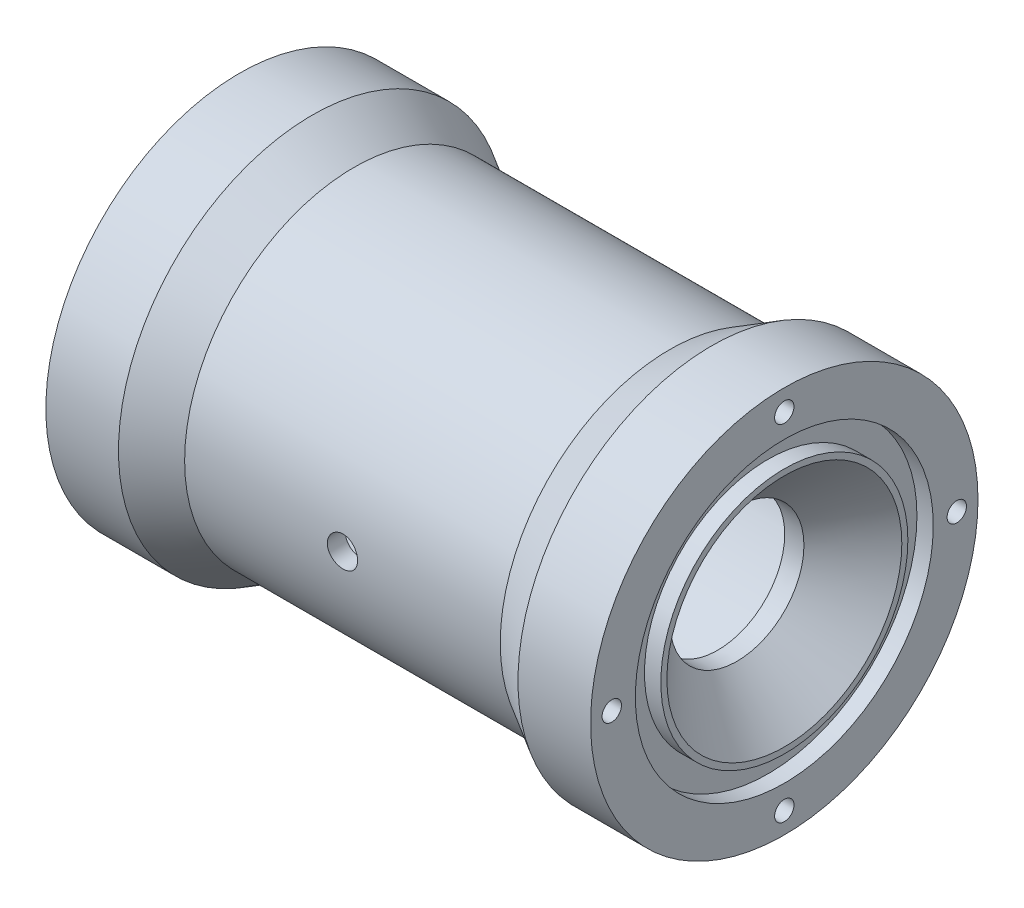
SolidWorks part; units mm, degrees
ref_plane "前视基准面" through (0, 0, 0) normal (0, 0, 1) x (1, 0, 0)
ref_plane "上视基准面" through (0, 0, 0) normal (0, 1, 0) x (1, 0, 0)
ref_plane "右视基准面" through (0, 0, 0) normal (1, 0, 0) x (0, 0, -1)
sketch "草图1" plane through (0, 0, 0) normal (0, 0, 1) x (1, 0, 0)
  line L0 (16.5, 16) -> (13.0359, 14)
  line L1 (22.4976, 16) -> (16.5, 16)
  line L2 (13.0359, 14) -> (-13.0359, 14)
  line L3 (-13.0359, 14) -> (-16.5, 16)
  line L4 (-16.5, 16) -> (-22.5, 16)
  line L5 (22.4976, 16) -> (22.4976, 12.3038)
  line L6 (22.4976, 12.3038) -> (21.1514, 12.3038)
  line L7 (21.1514, 12.3038) -> (21.1514, 10.2038)
  line L8 (21.1514, 10.2038) -> (22.5016, 10.2038)
  line L9 (22.5016, 10.2038) -> (22.5019, 9.7038)
  line L10 (22.5019, 9.7038) -> (18.5923, 5.5284)
  line L11 (18.5923, 5.5284) -> (17.0048, 5.5273)
  line L12 (17.0048, 5.5273) -> (17, 12.5)
  line L13 (17, 12.5) -> (-22.5, 12.5)
  line L14 (-22.5, 12.5) -> (-22.5, 16)
  line L15 (22.5, 0) -> (-22.5, 0) construction
revolve "旋转1" add sketch "草图1" angle 360 about L15
hole_wizard "M2 螺纹孔1" positions "草图2" profile "草图3" tap size "M2" standard "GB"
sketch "草图2" plane through (22.4976, 0, 0) normal (1, 0, 0) x (0, 0, -1)
  point P0 (0, 14.25)
  point P8 (14.25, 0)
  point P9 (0, -14.25)
  point P10 (-14.25, 0)
  point P11 (0, 0)
  dimension "D1" = 14.25
  dimension "D2" = 4
sketch "草图3" plane through (22.4976, 14.25, 0) normal (0, 1, 0) x (0, 0, -1)
  line L0 (0, 0) -> (0, 5.4807)
  line L1 (0, 5.4807) -> (0.8, 5)
  line L2 (0.8, 5) -> (0.8, 0)
  line L5 (0.8, 0) -> (0, 0)
  line L10 (0, 5.4807) -> (-0.8, 5) construction
  line L11 (0, -6.35) -> (0, 107.95) construction
  dimension "螺纹孔钻头直径" = 1.6
  dimension "螺纹孔钻头深度" = 5
  dimension "导头角度" = 118
cosmetic thread "孔螺蚊线1" parameters "D1"=4, "D2"=2
cosmetic thread "孔螺蚊线2" parameters "D1"=4, "D2"=2
cosmetic thread "孔螺蚊线3" parameters "D1"=4, "D2"=2
cosmetic thread "孔螺蚊线4" parameters "D1"=4, "D2"=2
hole_wizard "M2 螺纹孔2" positions "草图4" profile "草图5" tap size "M2" standard "GB"
sketch "草图4" plane through (-22.5, 0, 0) normal (-1, 0, 0) x (0, 0, 1)
  point P0 (0, 14.25)
  point P7 (14.25, 0)
  point P8 (0, -14.25)
  point P9 (-14.25, 0)
  point P10 (0, 0)
  dimension "D1" = 4
sketch "草图5" plane through (-22.5, 14.25, 0) normal (0, 1, 0) x (0, 0, 1)
  line L0 (0, 0) -> (0, 5.6807)
  line L1 (0, 5.6807) -> (0.8, 5.2)
  line L2 (0.8, 5.2) -> (0.8, 0)
  line L5 (0.8, 0) -> (0, 0)
  line L10 (0, 5.6807) -> (-0.8, 5.2) construction
  line L11 (0, -6.35) -> (0, 107.95) construction
  dimension "螺纹孔钻头直径" = 1.6
  dimension "螺纹孔钻头深度" = 5.2
  dimension "导头角度" = 118
cosmetic thread "孔螺蚊线5" parameters "D1"=4, "D2"=2
cosmetic thread "孔螺蚊线6" parameters "D1"=4, "D2"=2
cosmetic thread "孔螺蚊线7" parameters "D1"=4, "D2"=2
cosmetic thread "孔螺蚊线8" parameters "D1"=4, "D2"=2
sketch "草图9" plane through (0, 0, 0) normal (0, 0, 1) x (1, 0, 0)
  circle A0 centre (0, 0) radius 1.25
  dimension "D1" = 2.5
extrude "切除-拉伸1" cut sketch "草图9" along normal blind 20
cosmetic thread "装饰螺纹线1" parameters "D2"=3
